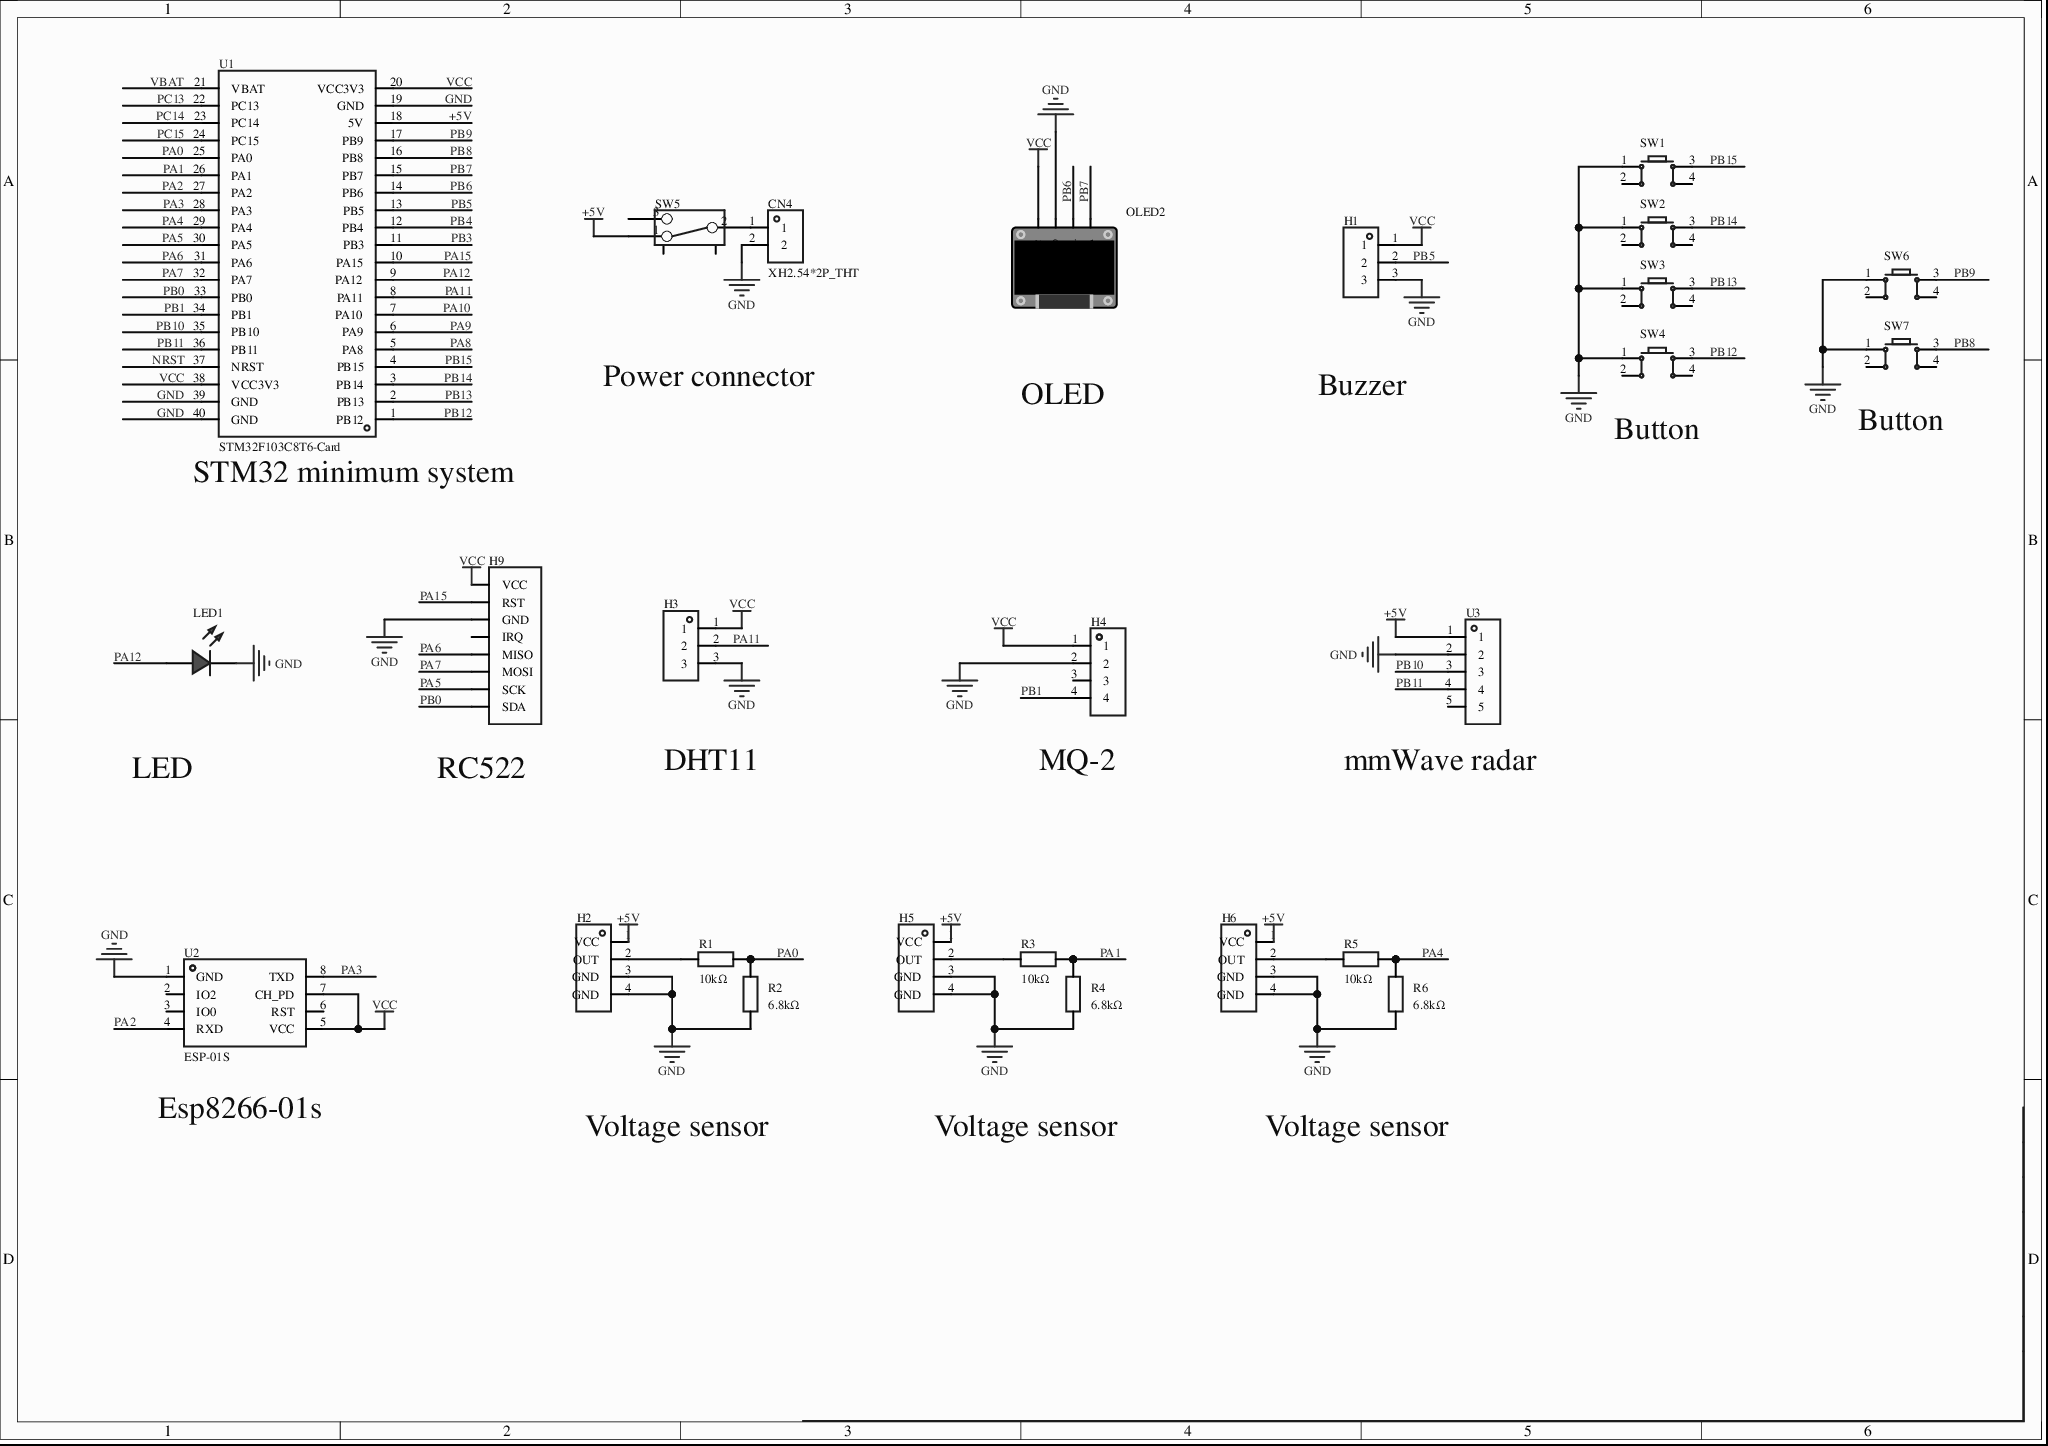
[diagram p0: MISC89009-3.schdoc]
# Altium project MISC89009-2.PrjPcb
1 sheet, 26 parts. Net scope: global (net labels, ports and power ports of the same name join across sheets).
Board file: MISC89009.pcbdoc

## Sheet MISC89009-3.schdoc
size 297 x 209 mm; Version: V1.0; @Project Name: MISC89009; @Page Count: 1; @Update Date: 2026-05-10; @Create Date: 2026-05-10; @Schematic Name: MISC89009; @Page No: 1; @Create Time: 23:22:16; @Update Time: 17:32:40; @Board Name: MISC89009

### Parts
CN4  XH2.54*2P_THT  [CONN-TH_2P-P2.50-XH2.54-2P]
H1  (no value)  [HDR-TH_3P-P2.54-V-F]
H2  (no value)  [HDR-TH_4P-P2.54-V-F]
H3  (no value)  [HDR-TH_3P-P2.54-V-F]
H4  (no value)  [HDR-TH_4P-P2.54-V-F]
H5  (no value)  [HDR-TH_4P-P2.54-V-F]
H6  (no value)  [HDR-TH_4P-P2.54-V-F]
H9  (no value)  [HDR-TH_8P-P2.54-V-F-1]
LED1  (no value)  [LED_TH-3mm]
OLED2  (no value)  [0.96OLED_4P]
R1  10kΩ  [Res_1/8W]
R2  6.8kΩ  [Res_1/8W]
R3  10kΩ  [Res_1/8W]
R4  6.8kΩ  [Res_1/8W]
R5  10kΩ  [Res_1/8W]
R6  6.8kΩ  [Res_1/8W]
SW1  (no value)  [SW-TH_4P-L6.0-W6.0-P4.50-LS6.5]
SW2  (no value)  [SW-TH_4P-L6.0-W6.0-P4.50-LS6.5]
SW3  (no value)  [SW-TH_4P-L6.0-W6.0-P4.50-LS6.5]
SW4  (no value)  [SW-TH_4P-L6.0-W6.0-P4.50-LS6.5]
SW5  (no value)  [拨动开关]
SW6  (no value)  [SW-TH_4P-L6.0-W6.0-P4.50-LS6.5]
SW7  (no value)  [SW-TH_4P-L6.0-W6.0-P4.50-LS6.5]
U1  STM32F103C8T6-Card  [CONN-TH_L53.3-W22.9_STM32F103C8T6-CARD]
U2  ESP-01S  [WIFIM-TH_ESP-01S]
U3  FPH12728-S05S1014190140B  [HDR-TH_5P-P1.27-V-M-1]  (value not drawn)

### Nets
+5V: H2.1(VCC) H5.1(VCC) H6.1(VCC) SW5.1 U1.18(5V) U3.1
GND: CN4.2 H1.3 H2.3(GND) H2.4(GND) H3.3 H4.2 H5.3(GND) H5.4(GND) H6.3(GND) H6.4(GND) H9.3(GND) LED1.2(A) OLED2.2(GND) R2.1 R4.1 R6.1 SW1.1 SW2.1 SW3.1 SW4.1 SW6.1 SW7.1 U1.19(GND) U1.39(GND) U1.40(GND) U2.1(GND) U3.2
VCC: H1.1 H3.1 H4.1 H9.1(VCC) OLED2.1(VCC) U1.20(VCC3V3) U1.38(VCC3V3) U2.5(VCC) U2.7(CH_PD)
NRST: U1.37(NRST)
PA0: R1.2 R2.2 U1.25(PA0)
PA1: R3.2 R4.2 U1.26(PA1)
PA2: U1.27(PA2) U2.4(RXD)
PA3: U1.28(PA3) U2.8(TXD)
PA4: R5.2 R6.2 U1.29(PA4)
PA5: H9.7(SCK) U1.30(PA5)
PA6: H9.5(MISO) U1.31(PA6)
PA7: H9.6(MOSI) U1.32(PA7)
PA8: U1.5(PA8)
PA9: U1.6(PA9)
PA10: U1.7(PA10)
PA11: H3.2 U1.8(PA11)
PA12: LED1.1(C) U1.9(PA12)
PA15: H9.2(RST) U1.10(PA15)
PB0: H9.8(SDA) U1.33(PB0)
PB1: H4.4 U1.34(PB1)
PB3: U1.11(PB3)
PB4: U1.12(PB4)
PB5: H1.2 U1.13(PB5)
PB6: OLED2.3(SCL) U1.14(PB6)
PB7: OLED2.4(SDA) U1.15(PB7)
PB8: SW7.3 U1.16(PB8)
PB9: SW6.3 U1.17(PB9)
PB10: U1.35(PB10) U3.3
PB11: U1.36(PB11) U3.4
PB12: SW4.3 U1.1(PB12)
PB13: SW3.3 U1.2(PB13)
PB14: SW2.3 U1.3(PB14)
PB15: SW1.3 U1.4(PB15)
PC13: U1.22(PC13)
PC14: U1.23(PC14)
PC15: U1.24(PC15)
VBAT: U1.21(VBAT)
NetCN4_1: CN4.1 SW5.2
NetH2_2: H2.2(OUT) R1.1
NetH5_2: H5.2(OUT) R3.1
NetH6_2: H6.2(OUT) R5.1

Not connected (* = marked no-connect by the designer): H4 3; H9 4(IRQ); SW1 2 4; SW2 2 4; SW3 2 4; SW4 2 4; SW5 3 4 5; SW6 2 4; SW7 2 4; U2 2(IO2)* 3(IO0)* 6(RST)*; U3 5

### Notes on the sheet
- Power connector
- OLED
- Buzzer
- (near SW7) Button
- (near U1) STM32 minimum system
- (near SW4) Button
- LED
- (near H9) RC522
- DHT11
- (near H4) MQ-2
- (near U3) mmWave radar
- (near U2) Esp8266-01s
- Voltage sensor

### Library data of the parts
CN4 = XH2.54*2P_直插: AddInBom: yes; ModelId: 325c595e30db4df8abe76612dd40b0fa0819f05c4eef4c71ace90d822a990e87; ModelTransform: 295.275,228.346,0,180,0,0,-0.002,-20.079,-137.795; Device: XH2.54*2P_THT; Symbol: XH2.54*2P_THT; FootprintName: CONN-TH_2P-P2.50-XH2.54-2P; LCSC Part Name: XH2.54*2P_直插; SupplierPart: C9900008615; ManufacturerPart: XH2.54*2P_直插; Supplier Footprint: XH2.54_2P; JLCPCB Part Class: Extended Part; Supplier: LCSC; ConvertToPcb: yes; ModelName: CONN-TH_2P-P2.50-XH2.54-2P
H1 H3 = HDR-F_2.54_1x3P: Symbol: PM254V-11-03-H85; ConvertToPcb: yes; ModelId: f3b3cc5aae9641bf9e56fc160cef875b; ModelName: HDR2.54-F-LI-1X3P; ModelTransform: 299.9994,100,0,0,0,0,0,0,-118.11; Device: HDR-F_2.54_1x3P; FootprintName: HDR-TH_3P-P2.54-V-F; AddInBom: yes; SupplierPart: C541850; Supplier Footprint: 插件
H2 = HDR-F_2.54_1x4P: Symbol: 2.54-1*4P female_1; ConvertToPcb: yes; ModelId: d187812051054f85879fcaa51a310d8e0819f05c4eef4c71ace90d822a990e87; ModelTransform: 419.6842,98.464,0,0,0,0,0,0,-118.11; Device: HDR-F_2.54_1x4P; AddInBom: yes; SupplierPart: C2718488; Supplier Footprint: 插件; FootprintName: HDR-TH_4P-P2.54-V-F; ModelName: HDR-TH_4P-P2.54-V-F
H4 = HDR-F_2.54_1x4P: Symbol: 2.54-1*4P female; ConvertToPcb: yes; ModelId: d187812051054f85879fcaa51a310d8e0819f05c4eef4c71ace90d822a990e87; ModelTransform: 419.6842,98.464,0,0,0,0,0,0,-118.11; Device: HDR-F_2.54_1x4P; FootprintName: HDR-TH_4P-P2.54-V-F; AddInBom: yes; SupplierPart: C2718488; Supplier Footprint: 插件; ModelName: HDR-TH_4P-P2.54-V-F
H5 H6 = HDR-F_2.54_1x4P: Symbol: 2.54-1*4P female_1; 3D Model: d187812051054f85879fcaa51a310d8e0819f05c4eef4c71ace90d822a990e87; 3D Model Transform: 419.6842,98.464,0,0,0,0,0,0,-118.11; ConvertToPcb: yes; Device: HDR-F_2.54_1x4P; Supplier Part: C2718488; Supplier Footprint: 插件; AddInBom: yes; FootprintName: HDR-TH_4P-P2.54-V-F; ModelName: HDR-TH_4P-P2.54-V-F
H9 = HDR-F_2.54_1x8P: Symbol: Header-Female-2.54_1x8_2; AddInBom: yes; ModelId: 0f7e4d9227ef4fa08d5469c22cc70cdb; ModelName: HDR-F-2.54_1x8; ModelTransform: 799.99844,100,0,0,0,0,0,0,-118.11; Device: HDR-F_2.54_1x8P; ConvertToPcb: yes; FootprintName: HDR-TH_8P-P2.54-V-F-1; SupplierPart: C27438; Supplier Footprint: 插件
LED1 = LED_TH-R_3mm: ConvertToPcb: yes; ModelId: a497c992633541038a38947cdc58012f0819f05c4eef4c71ace90d822a990e87; ModelName: LED-TH-3mm_R; ModelTransform: 141.274,153.327,0,0,0,0,-5.984,0,-137.795; Symbol: LED_TH-R; Device: LED_TH-R_3mm; AddInBom: yes; FootprintName: LED_TH-3mm; Supplier Footprint: 插件
OLED2 = 0.96OLED模块_4P: Symbol: 0.96OLED module_4P_1; Device: 0.96OLED module_4P; ConvertToPcb: yes; ModelId: 79c000fdb68d45a296c2e9bedf4f9055; ModelTransform: 1393.69792,1318.895,0,0,0,0,0,-560.079,-137.795; AddInBom: yes; FootprintName: 0.96OLED_4P; Supplier Footprint: 插件; ModelName: 0.96OLED_4P
R1-R6 = Res_AXIAL-1/8W: Symbol: Resistor; 3D Model: b2b5ae7ae4c642178fe0039925c86a3f0819f05c4eef4c71ace90d822a990e87; 3D Model Transform: 282.86,66.88,253.09,0,0,0,0,0,-191; ConvertToPcb: yes; ModelName: RES-TH_BD1.8-L3.2-P7.20-D0.4; Device: Res_AXIAL-1/8W; Supplier Footprint: 轴向引线; AddInBom: yes; FootprintName: Res_1/8W
  R1 R3 R5: Value: 10kΩ
  R2 R4 R6: Value: 6.8kΩ
SW1-SW4 = Key_TH_6x6x6: Contact current:50mA; Rated voltage (DC):12V; Insulation resistance:100MΩ; Circuit structure: SPST; Mounting: through-hole; Button shape: round; Button/cap colour: black; Actuation force: 260gf@±30gf; Operating temperature: -25℃~+70℃; Pin style: PC pin; Switch length: 6mm; Switch width: 6mm; Switch height: 6mm; With bracket: no;; Symbol: Tactile switch; AddInBom: yes; ModelId: 20eee248bc684ccd8cbdbb1d0d91ec6f0819f05c4eef4c71ace90d822a990e87; ModelName: SW-TH_4P-L6.0-W6.0-H5.0-LS6.5-P4.50; ModelTransform: 236.22,323.03,0,90,0,0,0,0,-137.795; Device: Key_TH_6x6x6; FootprintName: SW-TH_4P-L6.0-W6.0-P4.50-LS6.5; ConvertToPcb: yes; Supplier Footprint: 插件
SW5 = 拨动开关_正: Device: Toggle switch_pos; Symbol: Toggle switch; ConvertToPcb: yes; ModelId: 4321fe59a4074cbfb4989553f297c68f0819f05c4eef4c71ace90d822a990e87; ModelName: SW-TH_SS-12D02-VG4; ModelTransform: 370.09,208.7,472.35,0,0,0,0,0,-110; FootprintName: Toggle switch; AddInBom: yes; Supplier Footprint: 插件
SW6 SW7 = Key_TH_6x6x6: Contact current:50mA; Rated voltage (DC):12V; Insulation resistance:100MΩ; Circuit structure: SPST; Mounting: through-hole; Button shape: round; Button/cap colour: black; Actuation force: 260gf@±30gf; Operating temperature: -25℃~+70℃; Pin style: PC pin; Switch length: 6mm; Switch width: 6mm; Switch height: 6mm; With bracket: no;; Symbol: Tactile switch; 3D Model: 20eee248bc684ccd8cbdbb1d0d91ec6f0819f05c4eef4c71ace90d822a990e87; 3D Model Transform: 236.22,323.03,0,90,0,0,0,0,-137.795; AddInBom: yes; ModelName: SW-TH_4P-L6.0-W6.0-H5.0-LS6.5-P4.50; Device: Key_TH_6x6x6; Supplier Footprint: 插件; FootprintName: SW-TH_4P-L6.0-W6.0-P4.50-LS6.5; ConvertToPcb: yes
U1 = STM32F103C8T6-Card: AddInBom: yes; Device: STM32F103C8T6-Card; Symbol: STM32F103C8T6-CARD; FootprintName: CONN-TH_L53.3-W22.9_STM32F103C8T6-CARD; LCSC Part Name: STM32F103C8T6-Card; SupplierPart: C9900077949; ManufacturerPart: STM32F103C8T6-Card; Supplier Footprint: 插件; Supplier: LCSC; ConvertToPcb: yes
U2 = ESP-01S_C111009: AddInBom: yes; ModelId: eb7175da78ae48b3b1568cfe3027405f0819f05c4eef4c71ace90d822a990e87; ModelTransform: 582.676,976.37608,0,0,0,0,0,388.346,-118.11; Symbol: ESP-01S; Device: ESP-01S_C111009; LCSC Part Name: ESP-01S; SupplierPart: C111009; ManufacturerPart: ESP-01S; Supplier Footprint: -; JLCPCB Part Class: Extended Part; Supplier: LCSC; ConvertToPcb: yes; FootprintName: WIFIM-TH_ESP-01S; ModelName: WIFIM-TH_ESP-01S
U3 = FPH12728-S05S1014190140B: AddInBom: yes; ModelId: 092c149cf340410ca30a1e8c999c9f670819f05c4eef4c71ace90d822a990e87; ModelTransform: 250.393,94.488,0,0,0,0,0,0,-98.425; Symbol: FPH12728-S05S1014190140B; Device: FPH12728-S05S1014190140B; LCSC Part Name: FPH12728-S05S1014190140B; SupplierPart: C49253536; ManufacturerPart: FPH12728-S05S1014190140B; Supplier Footprint: 插件,P=1.27mm,5P; JLCPCB Part Class: Extended Part; Supplier: LCSC; ConvertToPcb: yes; FootprintName: HDR-TH_5P-P1.27-V-M-1; ModelName: HDR-TH_5P-P1.27-V-M-1